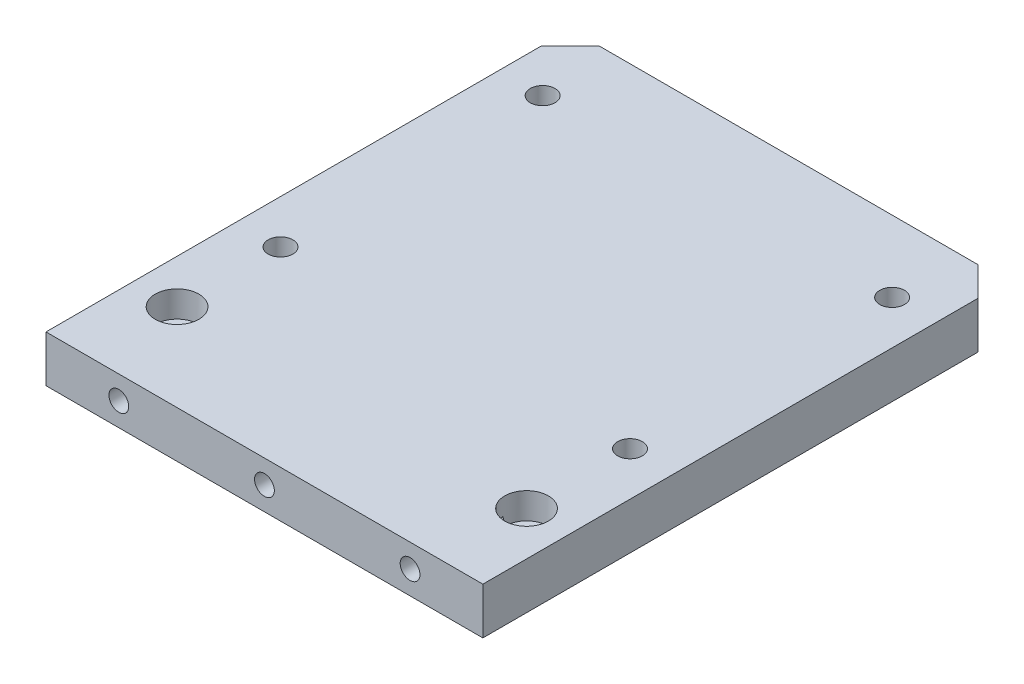
from build123d import *

# Parameters (mm, degrees)
SKETCH_1_W                = 150
SKETCH_1_H                = 180
EXTRUDE_1_DEPTH           = 16
HOLE_WIZARD_M8_1_D        = 6.8
HOLE_WIZARD_M8_1_DEPTH    = 29.25
HOLE_WIZARD_M8_1_TIP      = 2.042926105
HOLE_WIZARD_1_D           = 9
HOLE_WIZARD_1_DEPTH       = 29.25
HOLE_WIZARD_1_CBORE_D     = 15
HOLE_WIZARD_1_CBORE_DEPTH = 9
HOLE_WIZARD_1_TIP         = 2.703872786
HOLE_WIZARD_M10_1_D       = 8.5
CHAMFER_1_SIZE            = 10


with BuildPart() as part:
    # 草图1 → 凸台-拉伸1 (new body)
    with BuildSketch(Plane(origin=(0, 0, 0), x_dir=(1, 0, 0), z_dir=(0, 1, 0))):
        Rectangle(SKETCH_1_W, SKETCH_1_H)
    extrude(amount=EXTRUDE_1_DEPTH)

    # M8 螺纹孔1
    with Locations(Plane.XY.offset(90)):
        with Locations((-50, 8), (0, 8), (50, 8)):
            Hole(HOLE_WIZARD_M8_1_D / 2, depth=HOLE_WIZARD_M8_1_DEPTH)
            with Locations((0, 0, -(HOLE_WIZARD_M8_1_DEPTH + HOLE_WIZARD_M8_1_TIP / 2))):  # 118° drill point
                Cone(0, HOLE_WIZARD_M8_1_D / 2, HOLE_WIZARD_M8_1_TIP, mode=Mode.SUBTRACT)

    # 打孔尺寸(%根据)内六角圆柱头螺钉的类型1
    with Locations(Plane(origin=(0, 16, 0), x_dir=(1, 0, 0), z_dir=(0, 1, 0))):
        with Locations((-60, -60), (60, -60)):
            CounterBoreHole(HOLE_WIZARD_1_D / 2, HOLE_WIZARD_1_CBORE_D / 2, HOLE_WIZARD_1_CBORE_DEPTH, depth=HOLE_WIZARD_1_DEPTH)
            with Locations((0, 0, -(HOLE_WIZARD_1_DEPTH + HOLE_WIZARD_1_TIP / 2))):  # 118° drill point
                Cone(0, HOLE_WIZARD_1_D / 2, HOLE_WIZARD_1_TIP, mode=Mode.SUBTRACT)

    # M10 螺纹孔1 (through all)
    with Locations(Plane(origin=(0, 16, 0), x_dir=(1, 0, 0), z_dir=(0, 1, 0))):
        with Locations((-60, 65.51980275), (60, 65.51980275), (-60, -24.48019725), (60, -24.48019725)):
            Hole(HOLE_WIZARD_M10_1_D / 2)

    # 倒角1
    chamfer_1_edges = [part.edges().sort_by_distance(p)[0] for p in [
        (-75, 8, -90),
        (75, 8, -90),
    ]]
    chamfer(chamfer_1_edges, length=CHAMFER_1_SIZE)


solid = part.part
